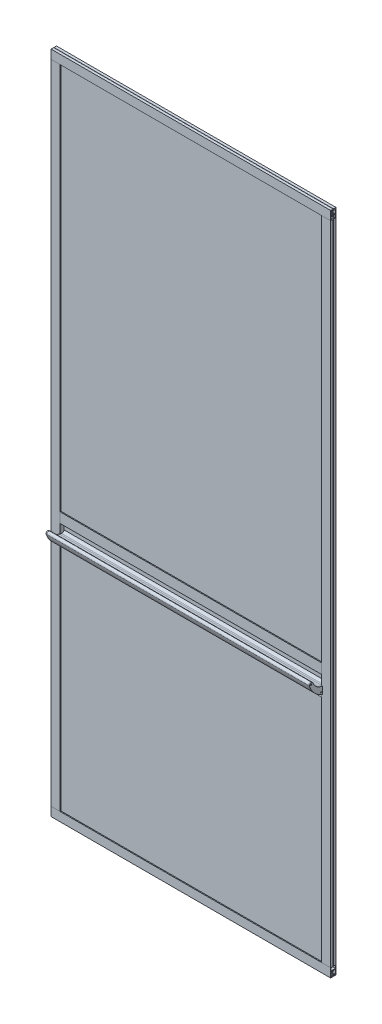
from build123d import *

# Parameters (mm, degrees)
D_XXXXXX_XX_XXXX_XXXX_XXXXXX_XXX_XXXXXXX_DEPTH = 940
D_XXXXXX_XX_XXXX_XXXX_XXXXXX_XXX_XXX_2_DEPTH   = 940
D_XXXXXX_XX_XXXX_XXXX_XXXXXX_XXX_XXX_3_DEPTH   = 2238
D_XXXXXX_XX_XXXX_XXXX_XXXXXX_XXX_XXX_5_DEPTH   = 2238
EXTRUDE_START                                  = -4
SKETCH_2_W                                     = 894
SKETCH_2_H                                     = 2190
EXTRUDE_1_DEPTH                                = 10
EXTRUDE_2_DEPTH                                = 880
CUT_EXTRUDE_2_DEPTH                            = 1447.942204502
CUT_EXTRUDE_2_DEPTH_BACK                       = 1447.942204502
SKETCH_5_W                                     = 10
SKETCH_5_H                                     = 80
SKETCH_6_R                                     = 2
EXTRUDE_3_DEPTH                                = 3
SKETCH_7_R                                     = 2
EXTRUDE_4_DEPTH                                = 2
SKETCH_8_R                                     = 2
EXTRUDE_5_DEPTH                                = 3


with BuildPart() as part:
    # Sketch1 → D_xxxxxx_xx_xxxx_xxxx_xxxxxx_xxx_xxxxxxx (new body)
    with BuildSketch(Plane(origin=(-470, 1118, 0), x_dir=(0, 0, -1), z_dir=(1, 0, 0))):
        with BuildLine():
            Line((-0.5, 0), (-9, 0))
            Line((-9, 0), (-9, -30))
            Line((-9, -30), (-5.9, -30))
            Line((-5.9, -30), (-5.9, -28.5))
            Line((-5.9, -28.5), (-7, -28.5))
            Line((-7, -28.5), (-7, -20))
            Line((-7, -20), (7, -20))
            Line((7, -20), (7, -28.5))
            Line((7, -28.5), (5.9, -28.5))
            Line((5.9, -28.5), (5.9, -30))
            Line((5.9, -30), (9, -30))
            Line((9, -30), (9, 0))
            Line((9, 0), (0.5, 0))
            ThreePointArc((0.5, 0), (0, -0.5), (-0.5, 0))
        make_face()
        with BuildLine():
            Line((-1.341640787, -3), (1.341640786, -3))
            ThreePointArc((1.341640786, -3), (1.799302724, -4.250096987), (1.272792206, -5.472792206))
            ThreePointArc((1.272792206, -5.472792206), (1.272792206, -6.250609665), (2.050609665, -6.250609665))
            ThreePointArc((2.050609665, -6.250609665), (2.853462499, -4.717447359), (2.640075756, -3))
            Line((2.640075756, -3), (7, -3))
            Line((7, -3), (7, -18))
            Line((7, -18), (2.640075756, -18))
            ThreePointArc((2.640075756, -18), (2.853462499, -16.282552641), (2.050609665, -14.749390335))
            ThreePointArc((2.050609665, -14.749390335), (1.272792206, -14.749390335), (1.272792206, -15.527207794))
            ThreePointArc((1.272792206, -15.527207794), (1.799302724, -16.749903013), (1.341640786, -18))
            Line((1.341640786, -18), (-1.341640787, -18))
            ThreePointArc((-1.341640787, -18), (-1.799302724, -16.749903013), (-1.272792206, -15.527207794))
            ThreePointArc((-1.272792206, -15.527207794), (-1.272792206, -14.749390335), (-2.050609665, -14.749390335))
            ThreePointArc((-2.050609665, -14.749390335), (-2.853462499, -16.282552641), (-2.640075756, -18))
            Line((-2.640075756, -18), (-7, -18))
            Line((-7, -18), (-7, -3))
            Line((-7, -3), (-2.640075756, -3))
            ThreePointArc((-2.640075756, -3), (-2.853462499, -4.717447359), (-2.050609665, -6.250609665))
            ThreePointArc((-2.050609665, -6.250609665), (-1.272792206, -6.250609665), (-1.272792206, -5.472792206))
            ThreePointArc((-1.272792206, -5.472792206), (-1.799302724, -4.250096987), (-1.341640787, -3))
        make_face(mode=Mode.SUBTRACT)
    extrude(amount=D_XXXXXX_XX_XXXX_XXXX_XXXXXX_XXX_XXXXXXX_DEPTH)


with BuildPart() as body_2:
    # Sketch1 on segment 2 (carried to segment 2) → D_xxxxxx_xx_xxxx_xxxx_xxxxxx_xxx_xxx 2 (new body)
    with BuildSketch(Plane(origin=(-470, -1118, 0), x_dir=(0, 0, 1), z_dir=(1, 0, 0))):
        with BuildLine():
            Line((-0.5, 0), (-9, 0))
            Line((-9, 0), (-9, -30))
            Line((-9, -30), (-5.9, -30))
            Line((-5.9, -30), (-5.9, -28.5))
            Line((-5.9, -28.5), (-7, -28.5))
            Line((-7, -28.5), (-7, -20))
            Line((-7, -20), (7, -20))
            Line((7, -20), (7, -28.5))
            Line((7, -28.5), (5.9, -28.5))
            Line((5.9, -28.5), (5.9, -30))
            Line((5.9, -30), (9, -30))
            Line((9, -30), (9, 0))
            Line((9, 0), (0.5, 0))
            ThreePointArc((0.5, 0), (0, -0.5), (-0.5, 0))
        make_face()
        with BuildLine():
            Line((-1.341640787, -3), (1.341640786, -3))
            ThreePointArc((1.341640786, -3), (1.799302724, -4.250096987), (1.272792206, -5.472792206))
            ThreePointArc((1.272792206, -5.472792206), (1.272792206, -6.250609665), (2.050609665, -6.250609665))
            ThreePointArc((2.050609665, -6.250609665), (2.853462499, -4.717447359), (2.640075756, -3))
            Line((2.640075756, -3), (7, -3))
            Line((7, -3), (7, -18))
            Line((7, -18), (2.640075756, -18))
            ThreePointArc((2.640075756, -18), (2.853462499, -16.282552641), (2.050609665, -14.749390335))
            ThreePointArc((2.050609665, -14.749390335), (1.272792206, -14.749390335), (1.272792206, -15.527207794))
            ThreePointArc((1.272792206, -15.527207794), (1.799302724, -16.749903013), (1.341640786, -18))
            Line((1.341640786, -18), (-1.341640787, -18))
            ThreePointArc((-1.341640787, -18), (-1.799302724, -16.749903013), (-1.272792206, -15.527207794))
            ThreePointArc((-1.272792206, -15.527207794), (-1.272792206, -14.749390335), (-2.050609665, -14.749390335))
            ThreePointArc((-2.050609665, -14.749390335), (-2.853462499, -16.282552641), (-2.640075756, -18))
            Line((-2.640075756, -18), (-7, -18))
            Line((-7, -18), (-7, -3))
            Line((-7, -3), (-2.640075756, -3))
            ThreePointArc((-2.640075756, -3), (-2.853462499, -4.717447359), (-2.050609665, -6.250609665))
            ThreePointArc((-2.050609665, -6.250609665), (-1.272792206, -6.250609665), (-1.272792206, -5.472792206))
            ThreePointArc((-1.272792206, -5.472792206), (-1.799302724, -4.250096987), (-1.341640787, -3))
        make_face(mode=Mode.SUBTRACT)
    extrude(amount=D_XXXXXX_XX_XXXX_XXXX_XXXXXX_XXX_XXX_2_DEPTH)


with BuildPart() as body_3:
    # Sketch1 on segment 3 (carried to segment 3) → D_xxxxxx_xx_xxxx_xxxx_xxxxxx_xxx_xxx 3 (new body)
    with BuildSketch(Plane(origin=(470, 1119, 0), x_dir=(0, 0, -1), z_dir=(0, -1, 0))):
        with BuildLine():
            Line((-0.5, 0), (-9, 0))
            Line((-9, 0), (-9, -30))
            Line((-9, -30), (-5.9, -30))
            Line((-5.9, -30), (-5.9, -28.5))
            Line((-5.9, -28.5), (-7, -28.5))
            Line((-7, -28.5), (-7, -20))
            Line((-7, -20), (7, -20))
            Line((7, -20), (7, -28.5))
            Line((7, -28.5), (5.9, -28.5))
            Line((5.9, -28.5), (5.9, -30))
            Line((5.9, -30), (9, -30))
            Line((9, -30), (9, 0))
            Line((9, 0), (0.5, 0))
            ThreePointArc((0.5, 0), (0, -0.5), (-0.5, 0))
        make_face()
        with BuildLine():
            Line((-1.341640787, -3), (1.341640786, -3))
            ThreePointArc((1.341640786, -3), (1.799302724, -4.250096987), (1.272792206, -5.472792206))
            ThreePointArc((1.272792206, -5.472792206), (1.272792206, -6.250609665), (2.050609665, -6.250609665))
            ThreePointArc((2.050609665, -6.250609665), (2.853462499, -4.717447359), (2.640075756, -3))
            Line((2.640075756, -3), (7, -3))
            Line((7, -3), (7, -18))
            Line((7, -18), (2.640075756, -18))
            ThreePointArc((2.640075756, -18), (2.853462499, -16.282552641), (2.050609665, -14.749390335))
            ThreePointArc((2.050609665, -14.749390335), (1.272792206, -14.749390335), (1.272792206, -15.527207794))
            ThreePointArc((1.272792206, -15.527207794), (1.799302724, -16.749903013), (1.341640786, -18))
            Line((1.341640786, -18), (-1.341640787, -18))
            ThreePointArc((-1.341640787, -18), (-1.799302724, -16.749903013), (-1.272792206, -15.527207794))
            ThreePointArc((-1.272792206, -15.527207794), (-1.272792206, -14.749390335), (-2.050609665, -14.749390335))
            ThreePointArc((-2.050609665, -14.749390335), (-2.853462499, -16.282552641), (-2.640075756, -18))
            Line((-2.640075756, -18), (-7, -18))
            Line((-7, -18), (-7, -3))
            Line((-7, -3), (-2.640075756, -3))
            ThreePointArc((-2.640075756, -3), (-2.853462499, -4.717447359), (-2.050609665, -6.250609665))
            ThreePointArc((-2.050609665, -6.250609665), (-1.272792206, -6.250609665), (-1.272792206, -5.472792206))
            ThreePointArc((-1.272792206, -5.472792206), (-1.799302724, -4.250096987), (-1.341640787, -3))
        make_face(mode=Mode.SUBTRACT)
    extrude(amount=D_XXXXXX_XX_XXXX_XXXX_XXXXXX_XXX_XXX_3_DEPTH)

    # D_xxxxxx_xx_xxxx_xxxx_xxxxxx_xxx_xxx 3 e
    split(bisect_by=Plane(origin=(470, 1088, 0), x_dir=(1, 0, 0), z_dir=(0, -1, 0)), keep=Keep.TOP)

    # D_xxxxxx_xx_xxxx_xxxx_xxxxxx_xxx_xxx 4
    split(bisect_by=Plane(origin=(470, -1088, 0), x_dir=(-1, 0, 0), z_dir=(0, 1, 0)), keep=Keep.TOP)


with BuildPart() as body_4:
    # Sketch1 on segment 4 (carried to segment 4) → D_xxxxxx_xx_xxxx_xxxx_xxxxxx_xxx_xxx 5 (new body)
    with BuildSketch(Plane(origin=(-470, 1119, 0), x_dir=(0, 0, 1), z_dir=(0, -1, 0))):
        with BuildLine():
            Line((-0.5, 0), (-9, 0))
            Line((-9, 0), (-9, -30))
            Line((-9, -30), (-5.9, -30))
            Line((-5.9, -30), (-5.9, -28.5))
            Line((-5.9, -28.5), (-7, -28.5))
            Line((-7, -28.5), (-7, -20))
            Line((-7, -20), (7, -20))
            Line((7, -20), (7, -28.5))
            Line((7, -28.5), (5.9, -28.5))
            Line((5.9, -28.5), (5.9, -30))
            Line((5.9, -30), (9, -30))
            Line((9, -30), (9, 0))
            Line((9, 0), (0.5, 0))
            ThreePointArc((0.5, 0), (0, -0.5), (-0.5, 0))
        make_face()
        with BuildLine():
            Line((-1.341640787, -3), (1.341640786, -3))
            ThreePointArc((1.341640786, -3), (1.799302724, -4.250096987), (1.272792206, -5.472792206))
            ThreePointArc((1.272792206, -5.472792206), (1.272792206, -6.250609665), (2.050609665, -6.250609665))
            ThreePointArc((2.050609665, -6.250609665), (2.853462499, -4.717447359), (2.640075756, -3))
            Line((2.640075756, -3), (7, -3))
            Line((7, -3), (7, -18))
            Line((7, -18), (2.640075756, -18))
            ThreePointArc((2.640075756, -18), (2.853462499, -16.282552641), (2.050609665, -14.749390335))
            ThreePointArc((2.050609665, -14.749390335), (1.272792206, -14.749390335), (1.272792206, -15.527207794))
            ThreePointArc((1.272792206, -15.527207794), (1.799302724, -16.749903013), (1.341640786, -18))
            Line((1.341640786, -18), (-1.341640787, -18))
            ThreePointArc((-1.341640787, -18), (-1.799302724, -16.749903013), (-1.272792206, -15.527207794))
            ThreePointArc((-1.272792206, -15.527207794), (-1.272792206, -14.749390335), (-2.050609665, -14.749390335))
            ThreePointArc((-2.050609665, -14.749390335), (-2.853462499, -16.282552641), (-2.640075756, -18))
            Line((-2.640075756, -18), (-7, -18))
            Line((-7, -18), (-7, -3))
            Line((-7, -3), (-2.640075756, -3))
            ThreePointArc((-2.640075756, -3), (-2.853462499, -4.717447359), (-2.050609665, -6.250609665))
            ThreePointArc((-2.050609665, -6.250609665), (-1.272792206, -6.250609665), (-1.272792206, -5.472792206))
            ThreePointArc((-1.272792206, -5.472792206), (-1.799302724, -4.250096987), (-1.341640787, -3))
        make_face(mode=Mode.SUBTRACT)
    extrude(amount=D_XXXXXX_XX_XXXX_XXXX_XXXXXX_XXX_XXX_5_DEPTH)

    # D_xxxxxx_xx_xxxx_xxxx_xxxxxx_xxx_xxx 5 e
    split(bisect_by=Plane(origin=(-470, 1088, 0), x_dir=(1, 0, 0), z_dir=(0, -1, 0)), keep=Keep.TOP)

    # D_xxxxxx_xx_xxxx_xxxx_xxxxxx_xxx_xxx 6
    split(bisect_by=Plane(origin=(-470, -1088, 0), x_dir=(-1, 0, 0), z_dir=(0, 1, 0)), keep=Keep.TOP)


with BuildPart() as body_5:
    # 草图2 → 凸台-拉伸1 (new body)
    with BuildSketch(Plane.XY.offset(9).offset(EXTRUDE_START)):
        Rectangle(SKETCH_2_W, SKETCH_2_H)
    extrude(amount=-EXTRUDE_1_DEPTH)

    # 草图5 → 切除-拉伸2 (cut, two sides: drawn at the far end of the back side and taken through both)
    with BuildSketch(Plane.ZY.offset(447).offset(-CUT_EXTRUDE_2_DEPTH_BACK)):
        with Locations((0, -265)):
            Rectangle(SKETCH_5_W, SKETCH_5_H)
    extrude(amount=CUT_EXTRUDE_2_DEPTH + CUT_EXTRUDE_2_DEPTH_BACK, mode=Mode.SUBTRACT)


with BuildPart() as body_6:
    # 草图4 → 凸台-拉伸2 (new body)
    with BuildSketch(Plane.ZY.offset(-440)):
        with BuildLine():
            Line((2.857553645, -247.108927406), (6.704462631, -245.385112329))
            ThreePointArc((6.704462631, -245.385112329), (6.919661361, -245.200645134), (7, -244.928828391))
            Line((7, -244.928828391), (7, -242.952423581))
            ThreePointArc((7, -242.952423581), (6.121320344, -240.831103238), (4, -239.952423581))
            Line((4, -239.952423581), (-4, -239.952423581))
            ThreePointArc((-4, -239.952423581), (-4.707106781, -240.2453168), (-5, -240.952423581))
            Line((-5, -240.952423581), (-5, -249.086015321))
            ThreePointArc((-5, -249.086015321), (-4.543633488, -249.925338042), (-3.591074738, -249.998583198))
            Line((-3.591074738, -249.998583198), (-3.347907918, -249.889619187))
            ThreePointArc((-3.347907918, -249.889619187), (-3.194897044, -249.885245411), (-3.08360929, -249.99034771))
            Line((-3.08360929, -249.99034771), (-2.895538614, -250.410050952))
            ThreePointArc((-2.895538614, -250.410050952), (-2.8816414, -250.529556054), (-2.938818386, -250.635411588))
            Line((-2.938818386, -250.635411588), (-3.678508693, -251.352733376))
            Line((-3.678508693, -251.352733376), (-3.596723641, -251.535246951))
            Line((-3.596723641, -251.535246951), (-3.140439702, -251.33078432))
            ThreePointArc((-3.140439702, -251.33078432), (-2.941801607, -251.350985338), (-2.859622684, -251.532951814))
            Line((-2.859622684, -251.532951814), (-3.131422947, -254.285427902))
            Line((-3.131422947, -254.285427902), (-5, -255.122744643))
            Line((-5, -255.122744643), (-5, -274.876431855))
            ThreePointArc((-5, -274.876431855), (-1.310885546, -278.990696117), (4, -280.517532911))
            Line((4, -280.517532911), (9, -280.517532911))
            ThreePointArc((9, -280.517532911), (29.001605349, -272.801616047), (41.658705692, -255.498512265))
            ThreePointArc((41.658705692, -255.498512265), (49.190680956, -252.177818295), (52.949400099, -259.50104779))
            ThreePointArc((52.949400099, -259.50104779), (36.94100116, -286.960097621), (10.522889115, -304.633569556))
            Line((10.522889115, -304.633569556), (9, -304.633569556))
            Line((9, -304.633569556), (9, -315))
            Line((9, -315), (5.9, -315))
            Line((5.9, -315), (5.9, -313.5))
            Line((5.9, -313.5), (7, -313.5))
            Line((7, -313.5), (7, -305))
            Line((7, -305), (-7, -305))
            Line((-7, -305), (-7, -313.5))
            Line((-7, -313.5), (-5.9, -313.5))
            Line((-5.9, -313.5), (-5.9, -315))
            Line((-5.9, -315), (-9, -315))
            Line((-9, -315), (-9, -305))
            Line((-9, -305), (-8.5, -304.5))
            Line((-8.5, -304.5), (-8.5, -302.5))
            Line((-8.5, -302.5), (-9, -302))
            Line((-9, -302), (-9, -228))
            Line((-9, -228), (-8.5, -227.5))
            Line((-8.5, -227.5), (-8.5, -225.5))
            Line((-8.5, -225.5), (-9, -225))
            Line((-9, -225), (-9, -215))
            Line((-9, -215), (-5.9, -215))
            Line((-5.9, -215), (-5.9, -216.5))
            Line((-5.9, -216.5), (-7, -216.5))
            Line((-7, -216.5), (-7, -225))
            Line((-7, -225), (7, -225))
            Line((7, -225), (7, -216.5))
            Line((7, -216.5), (5.9, -216.5))
            Line((5.9, -216.5), (5.9, -215))
            Line((5.9, -215), (9, -215))
            Line((9, -215), (9, -248.849289471))
            Line((9, -248.849289471), (6.9068237, -249.78725002))
            Line((6.9068237, -249.78725002), (5.994255823, -250.196175282))
            Line((5.994255823, -250.196175282), (3.759062035, -248.567093108))
            ThreePointArc((3.759062035, -248.567093108), (3.677947451, -248.384649697), (3.795076163, -248.222952329))
            Line((3.795076163, -248.222952329), (4.251360101, -248.018489698))
            Line((4.251360101, -248.018489698), (4.169575049, -247.835976122))
            Line((4.169575049, -247.835976122), (3.141897681, -247.910618755))
            ThreePointArc((3.141897681, -247.910618755), (3.024838296, -247.882839225), (2.944895799, -247.792929275))
            Line((2.944895799, -247.792929275), (2.756825122, -247.373226034))
            ThreePointArc((2.756825122, -247.373226034), (2.752451346, -247.220215159), (2.857553645, -247.108927406))
        make_face()
        with BuildLine():
            Line((-0.591607978, -302), (0.591607978, -302))
            ThreePointArc((0.591607978, -302), (1.754528537, -300.702031856), (1.272792206, -299.027207794))
            ThreePointArc((1.272792206, -299.027207794), (1.272792206, -298.249390335), (2.050609665, -298.249390335))
            ThreePointArc((2.050609665, -298.249390335), (2.8908371, -300.069650561), (2.349468025, -302))
            Line((2.349468025, -302), (7, -302))
            Line((7, -302), (7, -282.517532911))
            Line((7, -282.517532911), (4, -282.517532911))
            ThreePointArc((4, -282.517532911), (-1.098439293, -281.380585741), (-5.230769231, -278.185185708))
            ThreePointArc((-5.230769231, -278.185185708), (-6.33968311, -277.883616831), (-7, -278.824156774))
            Line((-7, -278.824156774), (-7, -302))
            Line((-7, -302), (-2.349468025, -302))
            ThreePointArc((-2.349468025, -302), (-2.890837099, -300.069650561), (-2.050609666, -298.249390335))
            ThreePointArc((-2.050609666, -298.249390335), (-1.272792206, -298.249390335), (-1.272792206, -299.027207794))
            ThreePointArc((-1.272792206, -299.027207794), (-1.754528537, -300.702031855), (-0.591607978, -302))
        make_face(mode=Mode.SUBTRACT)
        with BuildLine():
            Line((-2.349468025, -228), (-7, -228))
            Line((-7, -228), (-7, -237.952423581))
            Line((-7, -237.952423581), (7, -237.952423581))
            Line((7, -237.952423581), (7, -228))
            Line((7, -228), (2.349468025, -228))
            ThreePointArc((2.349468025, -228), (2.890837099, -229.930349439), (2.050609665, -231.750609665))
            ThreePointArc((2.050609665, -231.750609665), (1.272792206, -231.750609665), (1.272792206, -230.972792206))
            ThreePointArc((1.272792206, -230.972792206), (1.754528537, -229.297968144), (0.591607978, -228))
            Line((0.591607978, -228), (-0.591607978, -228))
            ThreePointArc((-0.591607978, -228), (-1.754528537, -229.297968144), (-1.272792206, -230.972792206))
            ThreePointArc((-1.272792206, -230.972792206), (-1.272792206, -231.750609665), (-2.050609665, -231.750609665))
            ThreePointArc((-2.050609665, -231.750609665), (-2.8908371, -229.930349439), (-2.349468025, -228))
        make_face(mode=Mode.SUBTRACT)
        with BuildLine():
            Line((47.990278547, -260.512974914), (49.42470127, -260.93826723))
            ThreePointArc((49.42470127, -260.93826723), (49.72344908, -261.181787003), (49.760223756, -261.565453207))
            ThreePointArc((49.760223756, -261.565453207), (37.064728814, -284.546306856), (16.273739662, -300.57846193))
            ThreePointArc((16.273739662, -300.57846193), (15.889893701, -300.600604766), (15.603815834, -300.34372448))
            Line((15.603815834, -300.34372448), (14.904952734, -298.876313524))
            ThreePointArc((14.904952734, -298.876313524), (16.389996434, -297.529474766), (16.646469065, -295.541120868))
            ThreePointArc((16.646469065, -295.541120868), (15.98776331, -295.127470377), (15.574112819, -295.786176132))
            ThreePointArc((15.574112819, -295.786176132), (12.86209147, -297.711531202), (13.418348531, -294.432410889))
            ThreePointArc((13.418348531, -294.432410889), (13.831999022, -293.773705134), (13.173293267, -293.360054644))
            ThreePointArc((13.173293267, -293.360054644), (11.493703581, -294.45472716), (10.925592049, -296.377376042))
            Line((10.925592049, -296.377376042), (9.5, -296.377376042))
            ThreePointArc((9.5, -296.377376042), (9.146446609, -296.230929432), (9, -295.877376042))
            Line((9, -295.877376042), (9, -282.025929779))
            ThreePointArc((9, -282.025929779), (28.875214056, -274.716759873), (42.854511276, -258.809926508))
            ThreePointArc((42.854511276, -258.809926508), (43.15129036, -258.559946567), (43.537497896, -258.597516964))
            Line((43.537497896, -258.597516964), (44.790550315, -259.274708837))
            ThreePointArc((44.790550315, -259.274708837), (45.415980474, -259.180714504), (45.539471562, -258.560434108))
            ThreePointArc((45.539471562, -258.560434108), (47.83577205, -256.154388388), (47.913373649, -259.479449279))
            ThreePointArc((47.913373649, -259.479449279), (47.587164388, -260.023346665), (47.990278547, -260.512974914))
        make_face(mode=Mode.SUBTRACT)
    extrude(amount=EXTRUDE_2_DEPTH)


with BuildPart() as cut_extrude_2_piece_1:
    # of the separate pieces the step leaves, piece 1, a body of its own (cut_extrude_2_pieces)
    add(body_5.part.solids().sort_by_distance((-447, 1095, 5))[0])


with BuildPart() as cut_extrude_2_piece_2:
    # of the separate pieces the step leaves, piece 2, a body of its own (cut_extrude_2_pieces)
    add(body_5.part.solids().sort_by_distance((-447, -1095, 5))[0])


with BuildPart() as body_8:
    # 草图6 → 凸台-拉伸3 (new body)
    with BuildSketch(Plane.ZY.offset(440)):
        with BuildLine():
            Line((9.5, -304.633569556), (10.522889115, -304.633569556))
            ThreePointArc((10.522889115, -304.633569556), (36.94100116, -286.960097621), (52.949400099, -259.50104779))
            ThreePointArc((52.949400099, -259.50104779), (49.190680956, -252.177818295), (41.658705691, -255.498512265))
            ThreePointArc((41.658705691, -255.498512265), (29.200353014, -272.648317686), (9.5, -280.472796488))
            Line((9.5, -280.472796488), (9.5, -304.633569556))
        make_face()
        with Locations((47.185930191, -257.832990651)):
            Circle(SKETCH_6_R, mode=Mode.SUBTRACT)
        with Locations((13.819348054, -296.187175655)):
            Circle(SKETCH_6_R, mode=Mode.SUBTRACT)
    extrude(amount=EXTRUDE_3_DEPTH)


with BuildPart() as body_9:
    # 草图7 → 凸台-拉伸4 (new body)
    with BuildSketch(Plane.ZY.offset(440)):
        Polygon((-5.7, -228), (-5.7, -239.952423581), (-3.7, -239.952423581), (-3.7, -249.952423581), (-5.7, -249.952423581), (-5.7, -302), (-3.7, -304), (3.7, -304), (5.7, -302), (5.7, -249.952423581), (3.7, -249.952423581), (3.7, -239.952423581), (5.7, -239.952423581), (5.7, -228), (3.7, -226), (-3.7, -226), align=None)
        with Locations((0, -229.7)):
            Circle(SKETCH_7_R, mode=Mode.SUBTRACT)
        with Locations((0, -300.3)):
            Circle(SKETCH_7_R, mode=Mode.SUBTRACT)
    extrude(amount=EXTRUDE_4_DEPTH)


with BuildPart() as body_10:
    # 草图8 → 凸台-拉伸5 (new body)
    with BuildSketch(Plane.ZY.offset(442)):
        Polygon((-6.7, -228), (-6.7, -239.952423581), (-3.7, -239.952423581), (-3.7, -249.952423581), (-6.7, -249.952423581), (-6.7, -302), (-4.7, -304), (4.7, -304), (6.7, -302), (6.7, -249.952423581), (3.7, -249.952423581), (3.7, -239.952423581), (6.7, -239.952423581), (6.7, -228), (4.7, -226), (-4.7, -226), align=None)
        with Locations((0, -229.7)):
            Circle(SKETCH_8_R, mode=Mode.SUBTRACT)
        with Locations((0, -300.3)):
            Circle(SKETCH_8_R, mode=Mode.SUBTRACT)
    extrude(amount=EXTRUDE_5_DEPTH)


with BuildPart() as body_11:
    # 镜向1: mirrored copy
    add(body_8.part.mirror(Plane(origin=(0, 0, 0), x_dir=(0, 0, 1), z_dir=(1, 0, 0))))


with BuildPart() as body_12:
    # Mirror 1 2: mirrored copy
    add(body_9.part.mirror(Plane(origin=(0, 0, 0), x_dir=(0, 0, 1), z_dir=(1, 0, 0))))


with BuildPart() as body_13:
    # Mirror 1 3: mirrored copy
    add(body_10.part.mirror(Plane(origin=(0, 0, 0), x_dir=(0, 0, 1), z_dir=(1, 0, 0))))


solid = Compound([part.part, body_2.part, body_3.part, body_4.part, body_6.part, cut_extrude_2_piece_1.part, cut_extrude_2_piece_2.part, body_8.part, body_9.part, body_10.part, body_11.part, body_12.part, body_13.part])
